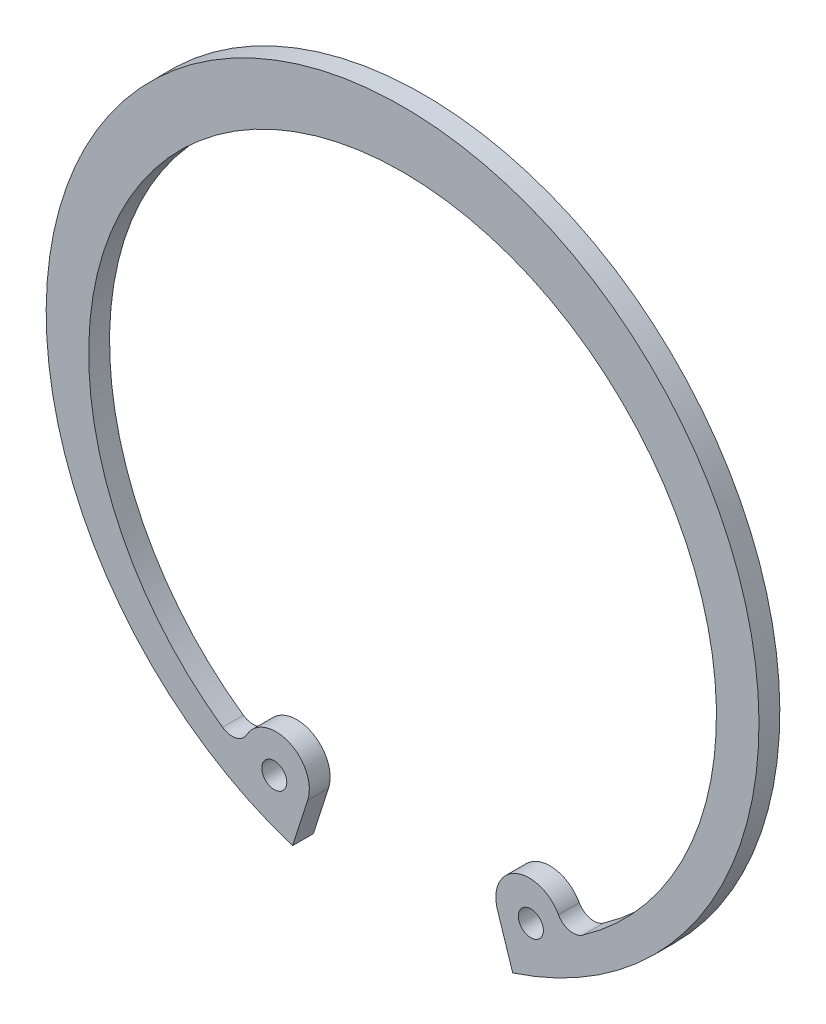
from build123d import *

# Parameters (mm, degrees)
EXTRUDE_962_DEPTH      = 1.25
EXTRUDE_962_DEPTH_BACK = 1.25
SKETCH_1_R             = 1.5


with BuildPart() as part:
    # 草图1 → Extrude 962 (new, two sides: drawn at the far end of the back side and taken through both)
    with BuildSketch(Plane.XY.offset(-EXTRUDE_962_DEPTH_BACK)):
        with BuildLine():
            Line((-11.382159751, -35.030685683), (-13.21047651, -40.657666072))
            ThreePointArc((-13.21047651, -40.657666072), (0, 42.75), (13.21047651, -40.657666072))
            Line((13.21047651, -40.657666072), (11.382159751, -35.030685683))
            ThreePointArc((11.382159751, -35.030685683), (13.598126255, -30.12345555), (18.691961025, -31.868237043))
            ThreePointArc((18.691961025, -31.868237043), (19.991161418, -32.852932397), (21.5917191, -32.543478506))
            ThreePointArc((21.5917191, -32.543478506), (0, 35.95), (-21.5917191, -32.543478506))
            ThreePointArc((-21.5917191, -32.543478506), (-19.991161418, -32.852932397), (-18.691961025, -31.868237043))
            ThreePointArc((-18.691961025, -31.868237043), (-13.598126255, -30.12345555), (-11.382159751, -35.030685683))
        make_face()
        with Locations((-15.388407261, -34.416375782)):
            Circle(SKETCH_1_R, mode=Mode.SUBTRACT)
        with Locations(Location((15.388407261, -34.416375782, 0), (0, 0, 180))):
            Circle(SKETCH_1_R, mode=Mode.SUBTRACT)
    extrude(amount=EXTRUDE_962_DEPTH + EXTRUDE_962_DEPTH_BACK)


solid = part.part
